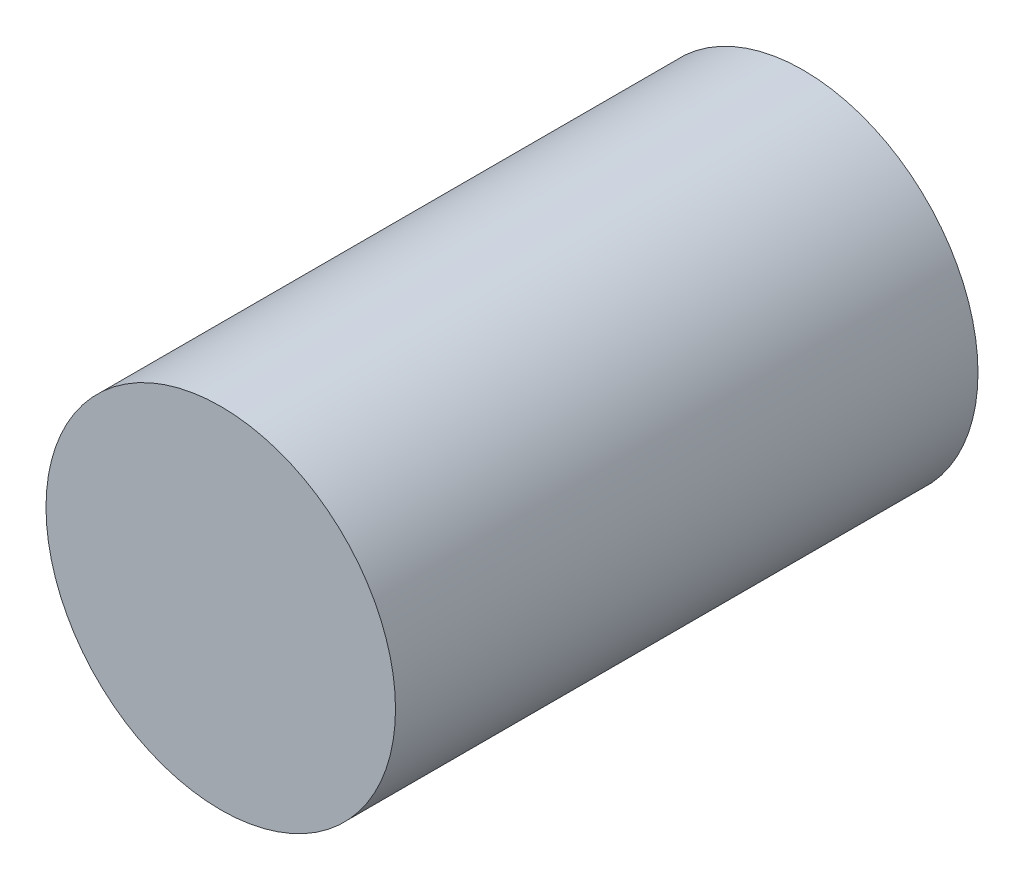
from build123d import *

# Parameters (mm, degrees)
SKETCH_1_R             = 7.5
EXTRUDE_1_DEPTH        = 25
HOLE_WIZARD_M4_1_D     = 3.3
HOLE_WIZARD_M4_1_DEPTH = 10.1
HOLE_WIZARD_M4_1_TIP   = 0.991420021


with BuildPart() as part:
    # 草图1 → 凸台-拉伸1 (new body)
    with BuildSketch(Plane.XY):
        Circle(SKETCH_1_R)
    extrude(amount=EXTRUDE_1_DEPTH)

    # M4 螺纹孔1
    with Locations(Plane(origin=(0, 0, 0), x_dir=(-1, 0, 0), z_dir=(0, 0, -1))):
        with Locations((0, 0)):
            Hole(HOLE_WIZARD_M4_1_D / 2, depth=HOLE_WIZARD_M4_1_DEPTH)
            with Locations((0, 0, -(HOLE_WIZARD_M4_1_DEPTH + HOLE_WIZARD_M4_1_TIP / 2))):  # 118° drill point
                Cone(0, HOLE_WIZARD_M4_1_D / 2, HOLE_WIZARD_M4_1_TIP, mode=Mode.SUBTRACT)


solid = part.part
